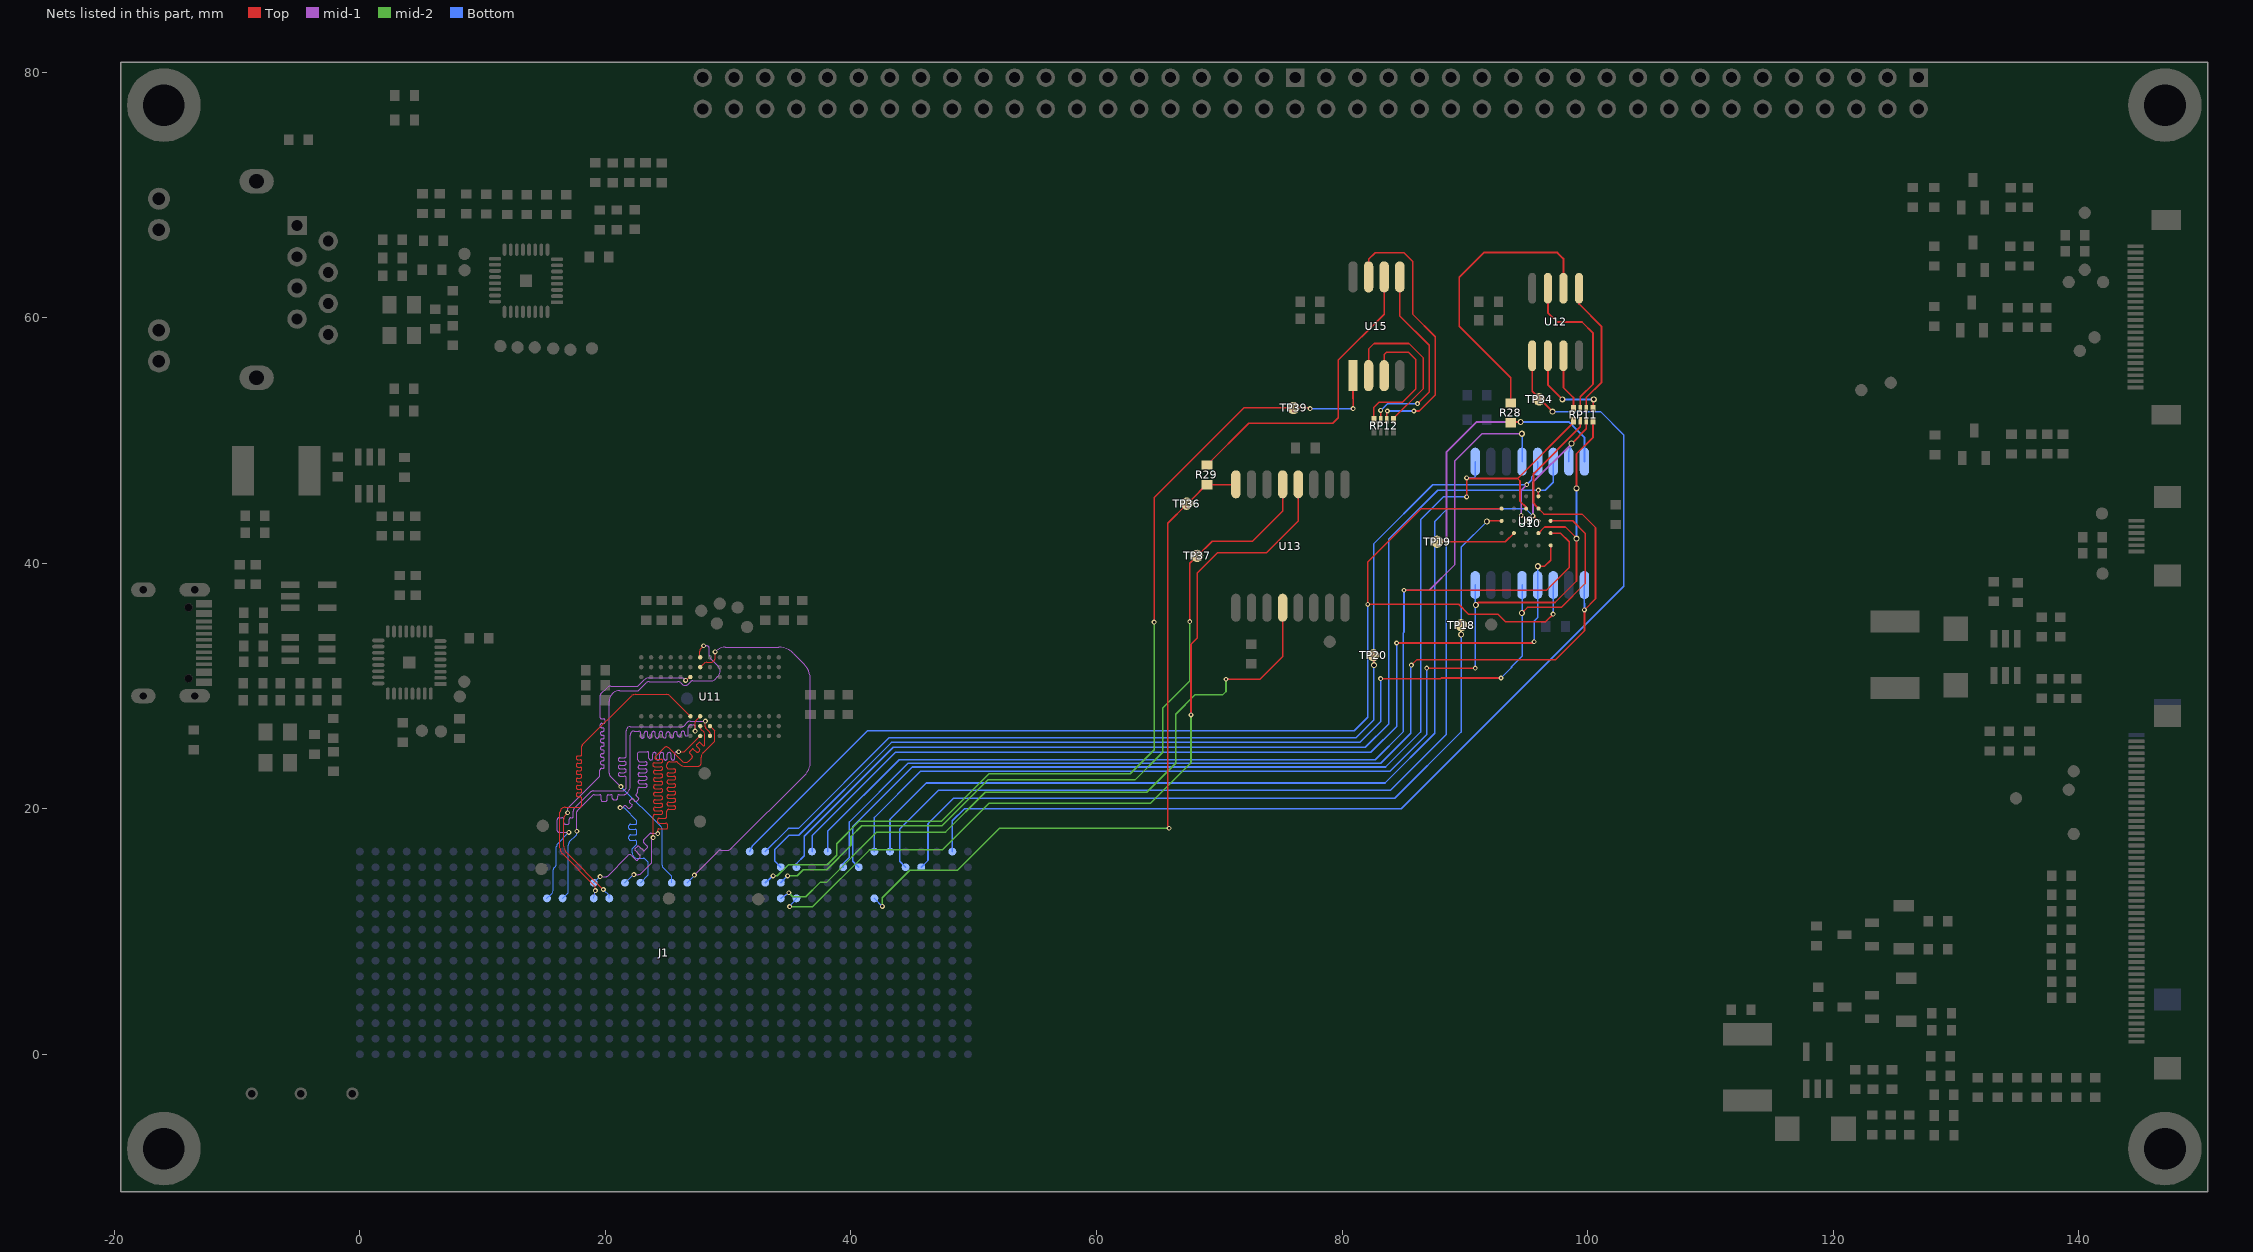
[diagram p0: the nets of this part, all layers, seen from the top]
# Altium PCB MISC105414.PcbDoc (part 8 of 11)
Units mm, origin at the board's own origin, x right, y up, seen from the top; angles counter-clockwise.
Board outline 170 x 92 mm, 6 copper layers (Top, GND, mid-1, mid-2, mid-3, Bottom), stack 1.231 mm thick; 238 components, 304 nets, 1456 pads, 1258 vias.
Unrouted connection lines stored in the file: 57.

## Via types
v1: diameter 0.4, hole 0.2, Top to Bottom, tented top, 618 vias
v2: diameter 0.5, hole 0.3, Top to Bottom, tented top, 522 vias
v3: diameter 0.5, hole 0.3, Top to Bottom, 41 vias
v4: diameter 1, hole 0.5, Top to Bottom, tented top, 36 vias
v5: diameter 0.7, hole 0.4, Top to Bottom, tented top, 34 vias
v6: diameter 1.3, hole 1.3, Top to Bottom, tented top, 3 vias
v7: diameter 4, hole 4, Top to Bottom, tented top, 2 vias
v8: diameter 3.3, hole 3.3, Top to Bottom, tented top, 2 vias

## Nets (pads, with @x,y where several pads share a name; then routed paths per layer and width w, separated by ;. In a path a pad name is that pad's centre, name@x,y a point inside that pad or via, vN(x,y) a via of type N, cw(c..) or ccw(c..) an arc to the next point about the centre after c; other vN are vias at no path point) (continued)
NOR_D6: J1.J12 U13.12 | length 67.1
  Top w0.127: v1(67.7,27.65) 67.7,33.4 68.2,33.9 68.2,39.2 69.85,40.85 73.85,40.85 76.435,43.435 U13.12@76.435,46.425
  mid-2 w0.127: v1(34.998,12.029) 36.886,12.029 41.504,16.648 47.446,16.648 51.246,20.447 64.397,20.447 67.7,23.75 v1(67.7,27.65)
  Bottom w0.127: v1(34.998,12.029) J1.J12@35.56,12.7
NOR_D7: J1.J13 U13.4 | length 56.2
  Top w0.127: v1(70.55,30.55) 73.315,30.55 75.165,32.4 U13.4@75.165,36.375
  mid-2 w0.127: v1(34.943,13.157) 35.265,12.835 36.323,12.835 37.485,13.997 38.006,13.997 42.109,18.1 47.7,18.1 50.947,21.347 64.097,21.347 66.45,23.7 66.45,27.7 68.05,29.3 70.3,29.3 70.55,29.55 v1(70.55,30.55)
  Bottom w0.127: J1.J13@34.29,12.7 v1(34.943,13.157)
NOR_DQS: J1.K13 TP37.1 U13.13 | length 63.8
  Top w0.127: v1(67.6,35.25) 67.6,40 TP37.1@68.2,40.6 68.227,40.6 69.427,41.8 72.715,41.8 75.165,44.25 U13.13@75.165,46.425
  mid-2 w0.127: v1(34.838,14.537) 35.619,14.537 36.124,15.042 38.024,15.042 40.006,17.024 40.006,17.75 40.881,18.625 47.425,18.625 51.147,22.347 63.147,22.347 65.4,24.6 65.4,28.2 67.6,30.4 v1(67.6,35.25)
  Bottom w0.127: J1.K13@34.29,13.97 v1(34.838,14.537)
NOR_SCLK: J1.J7 R29.2 TP36.1 U13.16 | length 59.6
  Top w0.127: v1(65.913,18.415) 65.913,18.489 65.8,18.602 65.8,43.251 67.375,44.825 67.75,45.201 ; TP36.1@67.35,44.85 67.701,45.201 67.75,45.201 ; U13.16@71.355,46.425 71.33,46.4 68.949,46.4 67.75,45.201
  mid-2 w0.127: v1(42.554,12.045) 42.554,12.759 44.79,14.995 48.688,14.995 52.108,18.415 v1(65.913,18.415)
  Bottom w0.127: J1.J7@41.91,12.7 v1(42.554,12.045)
NORE_CS: J1.K14 TP39.1 U15.1 | length 79.2
  Top w0.127: v1(64.7,35.2) 64.7,45.35 72,52.65 TP39.1@76.05,52.65 77.35,52.65 v1(77.4,52.6) ; U15.1@80.895,55.279 80.895,53.407 80.9,53.402 v1(80.9,52.6)
  mid-2 w0.127: v1(33.665,14.534) 33.993,14.534 34.904,15.445 38.068,15.445 38.839,16.216 38.839,17.15 40.664,18.975 47.375,18.975 51.247,22.847 62.747,22.847 64.7,24.8 v1(64.7,35.2)
  Bottom w0.127: J1.K14@33.02,13.97 v1(33.665,14.534) ; v1(77.4,52.6) v1(80.9,52.6)
NORE_D0: RP12.7 U15.5 | length 15.7
  Top w0.127: RP12.7@83.15,51.7 83.15,51.85 v1(83.15,52.45) ; U15.5@84.705,63.321 84.705,60.145 87.1,57.75 87.1,53.95 v1(86.15,53)
  Bottom w0.127: v1(83.15,52.45) 83.7,53 v1(86.15,53)
NORE_D1: RP12.5 U15.2 | length 13.3
  Top w0.127: U15.2@82.165,55.279 82.165,57.45 82.615,57.9 85.45,57.9 86.6,56.75 86.6,54.2 84.2,51.8 RP12.5@84.2,51.7
NORE_D2: RP12.8 U15.3 | length 12
  Top w0.127: RP12.8@82.6,51.7 82.6,52.7 83,53.1 84.9,53.1 86,54.2 86,56.6 85.4,57.2 83.635,57.2 83.435,57 U15.3@83.435,55.279
NORE_D3: RP12.6 U15.7 | length 22.4
  Top w0.127: U15.7@82.165,63.321 82.165,64.755 82.71,65.3 85.05,65.3 85.75,64.6 85.75,60.3 87.6,58.45 87.6,53.702 86.298,52.4 v1(85.85,52.4) ; RP12.6@83.65,51.7 83.65,52.4 v1(83.7,52.4)
  Bottom w0.127: v1(83.7,52.4) v1(85.85,52.4)
NORE_SCLK: R29.1 U15.6 | length 25.3
  Top w0.127: R29.1@69,48 72.4,51.4 79.25,51.4 79.7,51.85 79.7,56.55 83.435,60.285 U15.6@83.435,63.321
PS_CS: J1.L4 TP18.1 U9.A3 | length 70.3
  Top w0.127: v2(89.7,34.2) TP18.1@89.7,34.95 ; v2(91.8,43.4) 91.8,43.45 92.467,43.45 U9.A3@93,43.45
  Bottom w0.127: J1.L4@45.72,15.24 46.275,15.795 46.275,18.775 48.35,20.85 84.3,20.85 89.7,26.25 v2(89.7,34.2) 89.7,41.3 v2(91.8,43.4)
PS_D0: J1.M6 RP11.3 U9.D3 U10.15 | length 87.5
  Top w0.127: v1(95.55,43.85) U9.D3@96,43.45
  Top w0.15: v2(98.7,49.75) 99.9,50.95 RP11.3@99.9,51.6
  mid-1 w0.15: v1(95.55,43.85) 95.55,46.6 v2(98.7,49.75)
  Bottom w0.127: J1.M6@43.18,16.51 43.18,19.14 46.14,22.1 83.5,22.1 87.55,26.15 87.55,43.4 88.6,44.45 94.95,44.45 v1(95.55,43.85)
  Bottom w0.15: U10.15@98.475,48.275 98.475,49.037 v2(98.7,49.75)
PS_D1: J1.M7 RP11.4 U9.D2 U10.8 | length 93.1
  Top w0.127: v1(86.9,31.45) v1(90.85,31.45) ; v2(90.9,36.6) 91.1,36.8 97.35,36.8 99.1,38.55 v2(99.1,42) 99.1,42.05 98.2,42.95 96.5,42.95 U9.D2@96,42.45
  Top w0.15: v2(99.1,46.1) 99.1,48.9 100.45,50.25 RP11.4@100.45,51.6
  Bottom w0.127: J1.M7@41.91,16.51 41.91,19.292 45.668,23.05 83.9,23.05 86.9,26.05 v1(86.9,31.45) ; v1(90.85,31.45) 90.85,34.384 90.855,34.389 v2@90.855,36.6 ; U10.8@90.855,38.225 v2@90.855,36.6 ; v2(90.9,36.6) v2@90.855,36.6
  Bottom w0.15: v2(99.1,42) v2(99.1,46.1)
PS_D2: J1.L8 RP11.1 U9.C4 U10.9 | length 91.8
  Top w0.127: v1(90.15,45.4) v1(90.15,46.95) 90.2,46.9 94.3,46.9 94.5,46.7 94.5,45.05 95,44.55 U9.C4@95,44.45
  Top w0.15: 94.3,46.9 98.85,51.45 RP11.1@98.85,51.6
  Bottom w0.127: J1.L8@40.64,15.24 40.156,15.723 40.156,18.556 45,23.4 83.55,23.4 86.4,26.25 86.4,43.55 88.25,45.4 v1(90.15,45.4) ; v1(90.15,46.95) 90.75,46.95 90.855,47.05 U10.9@90.855,48.275
PS_D3: J1.L9 RP11.2 U9.D4 U10.1 | length 98.4
  Top w0.127: v1(85.65,31.7) 86.1,32.15 97.4,32.15 99.75,34.5 v1(99.75,36.2) 100.65,37.1 100.65,42.9 99.55,44 96.45,44 U9.D4@96,44.45
  Top w0.15: U9.D4@96,44.45 95.6,44.9 95.6,47.3 99.4,51.1 RP11.2@99.4,51.6
  Bottom w0.127: J1.L9@39.37,15.24 39.37,15.533 39.878,16.041 39.878,18.928 44.65,23.7 83.15,23.7 85.6,26.15 85.6,31.65 v1(85.65,31.7) ; U10.1@99.745,38.225 99.745,36.744 99.75,36.738 v1(99.75,36.2)
PS_D4: J1.L12 U9.D5 U10.14 | length 86.7
  Top w0.127: U9.D5@96,45.45 v1(96,45.95)
  Bottom w0.127: J1.L12@35.56,15.24 35.56,15.533 36.2,16.173 36.2,17.754 43.446,25 81.9,25 83.8,26.9 83.8,41.95 87.8,45.95 v1(96,45.95) 96.55,45.95 97.205,46.605 U10.14@97.205,48.275
PS_D5: J1.L13 U9.E3 U10.5 | length 90.4
  Top w0.127: v1(83.15,30.6) 88.025,30.6 88.075,30.65 v1(92.95,30.65) ; v2(94.65,35.95) 95.1,36.4 97.85,36.4 99.8,38.35 99.8,42.45 98.8,43.45 U9.E3@97,43.45
  Bottom w0.127: J1.L13@34.29,15.24 33.806,15.723 33.806,16.71 34.946,17.85 35.75,17.85 43.3,25.4 81.45,25.4 83.15,27.1 v1(83.15,30.6) ; v1(92.95,30.65) 93.807,31.507 93.807,31.557 94.665,32.415 v2@94.665,35.95 ; v2(94.65,35.95) v2@94.665,35.95 ; U10.5@94.665,38.225 v2@94.665,35.95
PS_D6: J1.M10 U9.E2 U10.12 | length 103.7
  Top w0.127: v1(85.05,37.8) 96.65,37.8 98.5,39.65 98.5,41.75 97.8,42.45 U9.E2@97,42.45
  mid-1 w0.127: v1(85.05,37.8) 87.1,37.8 89.2,39.9 89.2,48.35 91.4,50.55 v2(94.65,50.55)
  Bottom w0.127: J1.M10@38.1,16.51 38.1,18.175 43.925,24 82.7,24 85,26.3 85,34.35 85.05,34.4 v1(85.05,37.8) ; v2(94.65,50.55) 94.665,50.535 U10.12@94.665,48.275
PS_D7: J1.M11 U9.E1 U10.4 | length 79.4
  Top w0.127: v1(84.45,33.5) 95.55,33.5 v1(95.65,33.6) ; v2(95.95,39.75) 96.5,39.75 97,40.25 U9.E1@97,41.45
  Bottom w0.127: J1.M11@36.83,16.51 36.83,17.8 43.63,24.6 82.35,24.6 84.45,26.7 v1(84.45,33.5) ; v1(95.65,33.6) 95.65,35.299 95.935,35.583 95.935,38.987 v2(95.95,39.75)
PS_DQS: J1.M14 TP20.1 U9.C3 U10.13 | length 89.1
  Top w0.127: TP20.1@82.55,32.5 v2(82.6,31.7) ; v1(94.6,43.9) U9.C3@95,43.45
  mid-1 w0.127: v1(94.6,43.9) 94.6,45.95 v1(95.05,46.4)
  Bottom w0.127: J1.M14@33.02,16.51 34.91,18.4 35.725,18.4 43.125,25.8 81.15,25.8 82.6,27.25 v2(82.6,31.7) 82.6,41.6 87.4,46.4 v1(95.05,46.4) 95.45,46.8 95.45,47.028 95.935,47.513 U10.13@95.935,48.275
PS_RSTN: J1.M15 U9.A4 U10.3 | length 98.6
  Top w0.127: U9.A4@93,44.45 86.45,44.45 82.1,40.1 v1(82.1,36.65) 89.5,36.65 90.3,35.85 92.7,35.85 93.3,35.25 96.6,35.25 v1(97.2,35.85)
  Bottom w0.127: J1.M15@31.75,16.51 31.969,16.975 41.343,26.35 81,26.35 82.1,27.45 v1(82.1,36.65) ; v1(97.2,35.85) 97.2,36.564 97.205,36.568 U10.3@97.205,38.225
PS_SCLK: J1.L5 R28.2 TP19.1 U9.B2 U10.16 | length 96.2
  Top w0.127: v1(88.5,41.75) 93.3,41.75 U9.B2@94,42.45
  Top w0.15: TP19.1@87.75,41.75 v1(88.5,41.75) ; R28.2@93.75,51.45 93.75,51.5 v2(94.55,51.5)
  mid-1 w0.15: v1(88.5,41.75) 88.5,49.05 90.95,51.5 v2(94.55,51.5)
  Bottom w0.127: J1.L5@44.45,15.24 43.966,15.723 43.966,18.341 47.125,21.5 83.95,21.5 88.5,26.05 v1(88.5,41.75)
  Bottom w0.15: v2(94.55,51.5) 98.5,51.5 99.745,50.255 U10.16@99.745,48.275
PSE_CS: J1.M2 TP34.1 U12.1 | length 89.4
  Top w0.15: U12.1@95.495,56.9 95.495,54.005 TP34.1@96.15,53.35 ; TP34.1@96.05,53.35 TP34.1@96.15,53.35 ; v2(97.15,52.35) 96.5,53 TP34.1@96.15,53.35
  Bottom w0.127: J1.M2@48.26,16.51 48.26,19.019 49.241,20 84.825,20 102.95,38.125 102.95,50.45 101.05,52.35 v2(97.15,52.35)
PSE_D0: RP11.6 U12.5 | length 11.1
  Top w0.15: U12.5@99.305,62.4 99.305,61.122 101.15,59.277 101.15,54.75 99.9,53.5 RP11.6@99.9,52.6
PSE_D1: RP11.5 U12.2 | length 7.4
  Top w0.15: U12.2@96.765,56.9 96.765,54.535 v2(97.95,53.35) ; RP11.5@100.45,52.6 100.463,52.6 100.463,53.35 v2(100.5,53.35)
  Bottom w0.15: v2(97.95,53.35) v2(100.5,53.35)
PSE_D2: RP11.8 U12.3 | length 4.6
  Top w0.15: U12.3@98.035,56.9 98.035,54.315 98.85,53.5 RP11.8@98.85,52.6
PSE_D3: RP11.7 U12.7 | length 13
  Top w0.15: U12.7@96.765,62.4 96.765,60.4 97.515,59.65 99.55,59.65 100.45,58.75 100.45,54.6 99.4,53.55 RP11.7@99.4,52.6
PSE_SCLK: R28.1 U12.6 | length 23.9
  Top w0.15: R28.1@93.75,53.05 93.75,55.1 89.55,59.3 89.55,63.3 91.55,65.3 97.55,65.3 98.035,64.815 U12.6@98.035,62.4
SDR_A0: J1.K19 U11.G8 | length 32.5
  Top w0.1: U11.G8@27.72,31.533 28.017,31.83 cw(c28.253,31.595) 28.253,31.928 28.511,31.928 ccw(c28.511,32.41) 28.852,32.069 28.853,32.07 ccw(c28.657,32.267) 28.935,32.267 v1(28.935,32.781)
  mid-1 w0.1: v1(27.25,14.6) 29.204,16.554 cw(c29.397,16.362) 29.397,16.634 30.017,16.634 ccw(c30.017,16.854) 30.172,16.699 36.34,22.866 ccw(c35.522,23.684) 36.679,23.684 36.679,30.606 ccw(c35.03,30.606) 36.196,31.772 35.286,32.681 ccw(c34.103,31.498) 34.103,33.171 29.773,33.171 ccw(c29.773,32.091) 29.009,32.855 v1(28.935,32.781)
  Bottom w0.1: J1.K19@26.67,13.97 27.25,14.55 v1(27.25,14.6) v1@27.3,14.6
SDR_A1: J1.K20 U11.G9 | length 31.2
  Top w0.1: U11.G9@27.72,32.333 27.679,32.333 27.679,32.845 cw(c27.962,32.845) 27.762,33.044 v1(27.993,33.275)
  mid-1 w0.1: v1(21.266,21.808) 20.369,22.705 cw(c20.536,22.872) 20.3,22.872 20.3,28.759 cw(c21.154,28.759) 21.154,29.613 22.69,29.613 23.338,30.261 cw(c23.554,30.046) 23.554,30.351 25.91,30.351 cw(c25.91,30.032) 26.135,30.257 26.247,30.146 ccw(c26.449,30.348) 26.449,30.062 26.573,30.062 ccw(c26.573,30.254) 26.709,30.118 26.94,30.349 cw(c27.114,30.176) 27.114,30.421 28.619,30.421 ccw(c28.619,30.888) 28.949,30.558 29.166,30.776 ccw(c28.73,31.212) 29.347,31.212 ccw(c28.73,31.212) 29.166,31.648 28.594,32.22 cw(c28.893,32.518) 28.471,32.518 28.471,33.023 ccw(c28.219,33.023) 28.219,33.275 v1(27.993,33.275)
  Bottom w0.1: v1(21.266,21.808) 24.513,18.561 cw(c24.266,18.315) 24.615,18.315 24.615,15.418 ccw(c24.918,15.418) 24.703,15.204 25.365,14.543 cw(c25.28,14.458) 25.4,14.458 J1.K20@25.4,13.97
SDR_A2: J1.J24 U11.F7 | length 30.5
  Top w0.1: v1(16.923,19.672) 16.723,19.472 ccw(c17.03,19.164) 16.596,19.164 16.596,16.948 ccw(c17.275,16.948) 16.795,16.467 v1(19.84,13.422) ; v1(26.534,30.451) U11.F7@26.92,30.733
  mid-1 w0.1: v1(16.923,19.672) 16.923,20.007 cw(c16.987,20.007) 16.941,20.052 19.555,22.666 19.555,23.141 cw(c19.705,23.141) 19.705,23.291 19.774,23.291 ccw(c19.774,23.441) 19.924,23.441 ccw(c19.774,23.441) 19.774,23.591 19.733,23.591 cw(c19.733,23.741) 19.583,23.741 cw(c19.733,23.741) 19.733,23.891 19.774,23.891 ccw(c19.774,24.041) 19.924,24.041 ccw(c19.774,24.041) 19.774,24.191 19.733,24.191 cw(c19.733,24.341) 19.583,24.341 cw(c19.733,24.341) 19.733,24.491 19.774,24.491 ccw(c19.774,24.641) 19.924,24.641 ccw(c19.774,24.641) 19.774,24.791 19.733,24.791 cw(c19.733,24.941) 19.583,24.941 cw(c19.733,24.941) 19.733,25.091 19.774,25.091 ccw(c19.774,25.241) 19.924,25.241 ccw(c19.774,25.241) 19.774,25.391 19.733,25.391 cw(c19.733,25.541) 19.583,25.541 cw(c19.733,25.541) 19.733,25.691 19.774,25.691 ccw(c19.774,25.841) 19.924,25.841 ccw(c19.774,25.841) 19.774,25.991 19.733,25.991 cw(c19.733,26.141) 19.583,26.141 cw(c19.733,26.141) 19.733,26.291 19.774,26.291 ccw(c19.774,26.441) 19.924,26.441 ccw(c19.774,26.441) 19.774,26.591 19.733,26.591 cw(c19.733,26.741) 19.583,26.741 19.583,26.85 cw(c19.688,26.85) 19.688,26.955 19.849,26.955 ccw(c19.849,27.073) 19.966,27.073 19.966,27.221 ccw(c19.864,27.221) 19.864,27.324 19.672,27.324 cw(c19.672,27.413) 19.583,27.413 19.583,29.241 cw(c19.74,29.241) 19.629,29.352 20.133,29.856 cw(c20.44,29.55) 20.44,29.983 22.578,29.983 ccw(c22.578,30.118) 22.673,30.023 23.173,30.522 cw(c23.485,30.21) 23.485,30.652 26.234,30.652 cw(c26.234,30.431) 26.39,30.587 26.539,30.438 v1(26.534,30.451)
  Bottom w0.1: v1(19.84,13.422) 20.32,12.942 J1.J24@20.32,12.7
SDR_A3: J1.J25 U11.F3 | length 30.6
  Top w0.1: v1(19.19,13.334) 19.19,13.646 16.479,16.358 cw(c16.921,16.8) 16.295,16.8 16.295,19.697 cw(c16.72,19.697) 16.72,20.122 17.873,20.122 ccw(c17.873,20.316) 18.068,20.316 18.068,20.848 ccw(c17.918,20.848) 17.918,20.998 17.759,20.998 cw(c17.759,21.148) 17.609,21.148 cw(c17.759,21.148) 17.759,21.298 17.938,21.298 ccw(c17.938,21.448) 18.088,21.448 ccw(c17.938,21.448) 17.938,21.598 17.759,21.598 cw(c17.759,21.748) 17.609,21.748 cw(c17.759,21.748) 17.759,21.898 17.938,21.898 ccw(c17.938,22.048) 18.088,22.048 ccw(c17.938,22.048) 17.938,22.198 17.759,22.198 cw(c17.759,22.348) 17.609,22.348 cw(c17.759,22.348) 17.759,22.498 17.938,22.498 ccw(c17.938,22.648) 18.088,22.648 ccw(c17.938,22.648) 17.938,22.798 17.759,22.798 cw(c17.759,22.948) 17.609,22.948 cw(c17.759,22.948) 17.759,23.098 17.938,23.098 ccw(c17.938,23.248) 18.088,23.248 ccw(c17.938,23.248) 17.938,23.398 17.759,23.398 cw(c17.759,23.548) 17.609,23.548 cw(c17.759,23.548) 17.759,23.698 17.938,23.698 ccw(c17.938,23.848) 18.088,23.848 ccw(c17.938,23.848) 17.938,23.998 17.759,23.998 cw(c17.759,24.148) 17.609,24.148 cw(c17.759,24.148) 17.759,24.298 17.941,24.298 ccw(c17.941,24.448) 18.091,24.448 18.091,25.111 cw(c18.212,25.111) 18.126,25.197 22.113,29.184 cw(c22.416,28.88) 22.416,29.31 24.996,29.31 cw(c24.996,28.952) 25.248,29.205 U11.F3@26.92,27.533
  Bottom w0.1: J1.J25@19.05,12.7 v1(19.19,13.334)
SDR_A4: J1.K22 U11.G1 | length 31.6
  Top w0.1: v1(25.966,24.642) 26.429,24.642 U11.G1@27.72,25.933
  mid-1 w0.1: v1(21.201,20.086) 21.342,20.086 ccw(c21.342,20.179) 21.408,20.113 21.528,20.233 cw(c21.601,20.16) 21.674,20.233 21.853,20.055 ccw(c21.922,20.124) 21.991,20.055 22.169,20.233 ; 22.085,20.774 21.97,20.659 ccw(c22.045,20.584) 21.939,20.584 ccw(c22.045,20.584) 21.97,20.509 22.169,20.31 ; 22.085,20.774 cw(c22.167,20.691) 22.249,20.774 22.396,20.627 ccw(c22.48,20.71) 22.563,20.627 22.706,20.77 ccw(c22.653,20.822) 22.727,20.822 ccw(c22.653,20.822) 22.706,20.874 22.515,21.065 cw(c22.584,21.134) 22.486,21.134 cw(c22.584,21.134) 22.515,21.204 22.577,21.265 ccw(c22.482,21.36) 22.616,21.36 22.616,21.592 cw(c22.766,21.592) 22.766,21.742 23.253,21.742 ccw(c23.253,21.892) 23.403,21.892 ccw(c23.253,21.892) 23.253,22.042 22.803,22.042 cw(c22.803,22.192) 22.653,22.192 cw(c22.803,22.192) 22.803,22.342 23.253,22.342 ccw(c23.253,22.492) 23.403,22.492 ccw(c23.253,22.492) 23.253,22.642 22.803,22.642 cw(c22.803,22.792) 22.653,22.792 cw(c22.803,22.792) 22.803,22.942 23.253,22.942 ccw(c23.253,23.092) 23.403,23.092 ccw(c23.253,23.092) 23.253,23.242 22.803,23.242 cw(c22.803,23.392) 22.653,23.392 cw(c22.803,23.392) 22.803,23.542 23.253,23.542 ccw(c23.253,23.692) 23.403,23.692 ccw(c23.253,23.692) 23.253,23.842 22.803,23.842 cw(c22.803,23.992) 22.653,23.992 22.653,24.552 22.755,24.653 23.393,24.653 cw(c23.393,24.503) 23.543,24.503 23.543,24.121 ccw(c23.693,24.121) 23.843,24.121 23.843,24.436 cw(c23.993,24.436) 24.143,24.436 24.143,24.121 ccw(c24.293,24.121) 24.443,24.121 24.443,24.436 cw(c24.593,24.436) 24.743,24.436 24.743,24.121 ccw(c24.893,24.121) 25.043,24.121 25.043,24.436 cw(c25.193,24.436) 25.343,24.436 25.343,24.121 ccw(c25.493,24.121) 25.643,24.121 25.643,24.513 cw(c25.772,24.513) 25.772,24.642 v1(25.966,24.642) ; 22.169,20.233 ccw(c22.13,20.272) 22.185,20.272 ccw(c22.13,20.272) 22.169,20.31
  Bottom w0.1: v1(21.201,20.086) 21.416,20.086 cw(c21.416,19.879) 21.562,20.025 22.504,19.083 cw(c22.37,18.949) 22.56,18.949 22.56,18.849 cw(c22.447,18.849) 22.447,18.736 22.047,18.736 ccw(c22.047,18.604) 21.915,18.604 21.915,18.415 ccw(c22.017,18.415) 22.017,18.312 22.434,18.312 cw(c22.434,18.186) 22.56,18.186 22.56,17.983 cw(c22.447,17.983) 22.447,17.87 22.061,17.87 ccw(c22.061,17.724) 21.915,17.724 21.915,17.571 ccw(c22.065,17.571) 22.065,17.422 22.427,17.422 cw(c22.427,17.288) 22.56,17.288 22.56,17.226 cw(c22.305,17.226) 22.485,17.046 22.18,16.741 22.18,16.408 ccw(c22.613,16.408) 22.613,15.975 23.085,15.975 cw(c23.085,15.814) 23.2,15.928 23.423,15.704 cw(c23.238,15.519) 23.5,15.519 23.5,14.61 J1.K22@22.86,13.97
SDR_A5: J1.K23 U11.G2 | length 30.4
  Top w0.1: v1(23.889,17.647) 23.889,19.389 cw(c24.039,19.389) 24.039,19.539 24.52,19.539 ccw(c24.52,19.689) 24.67,19.689 ccw(c24.52,19.689) 24.52,19.839 24.061,19.839 cw(c24.061,19.989) 23.911,19.989 cw(c24.061,19.989) 24.061,20.139 24.52,20.139 ccw(c24.52,20.289) 24.67,20.289 ccw(c24.52,20.289) 24.52,20.439 24.061,20.439 cw(c24.061,20.589) 23.911,20.589 cw(c24.061,20.589) 24.061,20.739 24.52,20.739 ccw(c24.52,20.889) 24.67,20.889 ccw(c24.52,20.889) 24.52,21.039 24.061,21.039 cw(c24.061,21.189) 23.911,21.189 cw(c24.061,21.189) 24.061,21.339 24.52,21.339 ccw(c24.52,21.489) 24.67,21.489 ccw(c24.52,21.489) 24.52,21.639 24.061,21.639 cw(c24.061,21.789) 23.911,21.789 cw(c24.061,21.789) 24.061,21.939 24.52,21.939 ccw(c24.52,22.089) 24.67,22.089 ccw(c24.52,22.089) 24.52,22.239 24.061,22.239 cw(c24.061,22.389) 23.911,22.389 cw(c24.061,22.389) 24.061,22.539 24.52,22.539 ccw(c24.52,22.689) 24.67,22.689 ccw(c24.52,22.689) 24.52,22.839 24.061,22.839 cw(c24.061,22.989) 23.911,22.989 cw(c24.061,22.989) 24.061,23.139 24.52,23.139 ccw(c24.52,23.289) 24.67,23.289 ccw(c24.52,23.289) 24.52,23.439 23.994,23.439 cw(c23.994,23.589) 23.844,23.589 cw(c23.994,23.589) 23.994,23.739 24.52,23.739 ccw(c24.52,23.889) 24.67,23.889 ccw(c24.52,23.889) 24.52,24.039 24.153,24.039 cw(c24.153,24.161) 24.031,24.161 cw(c24.153,24.161) 24.067,24.247 24.777,24.958 cw(c24.966,24.769) 25.155,24.958 26.201,23.911 ccw(c26.519,24.23) 26.838,23.911 27.05,24.123 ccw(c26.941,24.232) 27.095,24.232 ccw(c26.941,24.232) 27.05,24.341 26.858,24.533 cw(c26.911,24.586) 26.836,24.586 cw(c26.911,24.586) 26.858,24.64 27.082,24.864 cw(c27.12,24.825) 27.159,24.864 ; 27.159,24.864 27.382,24.641 ccw(c27.489,24.748) 27.596,24.641 27.667,24.712 ccw(c27.595,24.785) 27.698,24.785 ccw(c27.595,24.785) 27.667,24.858 27.433,25.092 cw(c27.498,25.157) 27.406,25.157 cw(c27.498,25.157) 27.433,25.222 27.592,25.381 cw(c27.65,25.324) 27.707,25.381 27.923,25.165 ccw(c28.001,25.242) 28.11,25.242 28.11,26.001 ccw(c27.723,26.001) 27.997,26.275 27.78,26.492 cw(c27.925,26.637) 27.72,26.637 U11.G2@27.72,26.733
  mid-1 w0.1: v1(22.317,14.641) 22.676,14.641 ccw(c22.676,14.994) 22.925,14.744 23.734,15.554 ccw(c23.625,15.663) 23.78,15.663 23.78,17.538 v1(23.889,17.647)
  Bottom w0.1: J1.K23@21.59,13.97 22.137,14.517 v1(22.317,14.641)
SDR_A6: J1.J27 U11.G3 | length 31.5
  Top w0.1: v1(27.302,26.332) 27.302,27.052 cw(c27.452,27.052) 27.346,27.158 U11.G3@27.72,27.533
  mid-1 w0.1: v1(17.672,18.167) 17.672,19.753 cw(c17.807,19.753) 17.712,19.849 18.959,21.096 cw(c19.107,20.948) 19.107,21.157 19.549,21.157 cw(c19.549,21.063) 19.643,21.063 19.643,20.729 ccw(c19.771,20.729) 19.771,20.601 19.995,20.601 ccw(c19.995,20.748) 20.141,20.748 20.141,21.059 cw(c20.239,21.059) 20.239,21.157 20.446,21.157 cw(c20.446,21.042) 20.562,21.042 20.562,20.859 ccw(c20.67,20.859) 20.67,20.751 20.895,20.751 ccw(c20.895,20.851) 20.994,20.851 20.994,21.037 cw(c21.114,21.037) 21.114,21.157 21.521,21.157 ccw(c21.521,21.392) 21.687,21.226 21.862,21.401 ccw(c21.505,21.758) 22.01,21.758 22.01,25.997 cw(c22.345,25.997) 22.345,26.332 22.715,26.332 cw(c22.715,26.182) 22.865,26.182 22.865,25.907 ccw(c23.015,25.907) 23.165,25.907 23.165,26.144 cw(c23.315,26.144) 23.465,26.144 23.465,25.907 ccw(c23.615,25.907) 23.765,25.907 23.765,26.144 cw(c23.915,26.144) 24.065,26.144 24.065,25.907 ccw(c24.215,25.907) 24.365,25.907 24.365,26.144 cw(c24.515,26.144) 24.665,26.144 24.665,25.923 ccw(c24.815,25.923) 24.965,25.923 24.965,26.108 cw(c25.115,26.108) 25.265,26.108 25.265,25.923 ccw(c25.415,25.923) 25.565,25.923 25.565,26.135 cw(c25.715,26.135) 25.865,26.135 25.865,26.016 ccw(c26.015,26.016) 26.165,26.016 26.165,26.164 cw(c26.315,26.164) 26.465,26.164 26.465,26.077 ccw(c26.615,26.077) 26.765,26.077 26.765,26.627 cw(c26.903,26.627) 26.805,26.725 26.879,26.798 cw(c26.973,26.704) 26.973,26.837 27.203,26.837 cw(c27.203,26.739) 27.302,26.739 v1(27.302,26.332)
  Bottom w0.1: J1.J27@16.51,12.7 16.984,13.174 16.984,17.033 cw(c17.413,17.033) 17.11,17.336 17.608,17.834 ccw(c17.451,17.99) 17.672,17.99 v1(17.672,18.167)
SDR_A7: J1.J28 U11.H1 | length 31.8
  Top w0.1: v1(28.137,27.138) 28.137,26.677 ccw(c28.337,26.677) 28.195,26.535 28.479,26.251 cw(c28.381,26.152) 28.52,26.152 U11.H1@28.52,25.933
  mid-1 w0.1: v1(17.031,18.072) 16.226,18.072 cw(c16.226,18.216) 16.081,18.216 16.081,19.123 cw(c16.236,19.123) 16.236,19.278 16.456,19.278 cw(c16.456,19.13) 16.604,19.13 16.604,18.867 ccw(c16.721,18.867) 16.721,18.751 16.959,18.751 ccw(c16.959,18.841) 17.05,18.841 17.05,19.137 cw(c17.169,19.137) 17.169,19.255 17.279,19.255 ccw(c17.279,19.349) 17.372,19.349 17.372,19.816 cw(c17.664,19.816) 17.458,20.022 18.803,21.367 cw(c19.019,21.151) 19.019,21.457 21.39,21.457 ccw(c21.39,21.702) 21.563,21.529 21.654,21.619 ccw(c21.539,21.733) 21.701,21.733 21.701,22.502 ccw(c21.551,22.502) 21.551,22.652 21.198,22.652 cw(c21.198,22.802) 21.048,22.802 cw(c21.198,22.802) 21.198,22.952 21.547,22.952 ccw(c21.547,23.102) 21.697,23.102 ccw(c21.547,23.102) 21.547,23.252 21.198,23.252 cw(c21.198,23.402) 21.048,23.402 cw(c21.198,23.402) 21.198,23.552 21.547,23.552 ccw(c21.547,23.702) 21.697,23.702 ccw(c21.547,23.702) 21.547,23.852 21.198,23.852 cw(c21.198,24.002) 21.048,24.002 cw(c21.198,24.002) 21.198,24.152 21.547,24.152 ccw(c21.547,24.302) 21.697,24.302 21.697,26.352 cw(c22.033,26.352) 22.033,26.688 26.234,26.688 ccw(c26.234,26.954) 26.422,26.766 26.724,27.068 cw(c26.892,26.9) 26.892,27.138 v1(28.137,27.138)
  Bottom w0.1: J1.J28@15.24,12.7 15.622,13.082 ccw(c15.319,13.386) 15.748,13.386 15.748,15.046 cw(c15.983,15.046) 15.817,15.212 15.942,15.337 ccw(c15.768,15.511) 16.014,15.511 16.014,16.913 cw(c16.356,16.913) 16.114,17.155 v1(17.031,18.072)
SDR_A8: J1.K25 U11.H2 | length 30.9
  Top w0.1: v1(24.263,17.981) 24.263,18.262 cw(c24.364,18.262) 24.364,18.363 24.962,18.363 ccw(c24.962,18.464) 25.063,18.464 25.063,18.691 ccw(c24.924,18.691) 24.924,18.829 24.393,18.829 cw(c24.393,18.96) 24.263,18.96 24.263,19.113 cw(c24.388,19.113) 24.388,19.238 24.873,19.238 ccw(c24.873,19.37) 25.006,19.37 25.006,19.794 cw(c25.156,19.794) 25.156,19.944 25.58,19.944 ccw(c25.58,20.094) 25.73,20.094 ccw(c25.58,20.094) 25.58,20.244 25.16,20.244 cw(c25.16,20.394) 25.01,20.394 cw(c25.16,20.394) 25.16,20.544 25.58,20.544 ccw(c25.58,20.694) 25.73,20.694 ccw(c25.58,20.694) 25.58,20.844 25.16,20.844 cw(c25.16,20.994) 25.01,20.994 cw(c25.16,20.994) 25.16,21.144 25.58,21.144 ccw(c25.58,21.294) 25.73,21.294 ccw(c25.58,21.294) 25.58,21.444 25.16,21.444 cw(c25.16,21.594) 25.01,21.594 cw(c25.16,21.594) 25.16,21.744 25.58,21.744 ccw(c25.58,21.894) 25.73,21.894 ccw(c25.58,21.894) 25.58,22.044 25.16,22.044 cw(c25.16,22.194) 25.01,22.194 cw(c25.16,22.194) 25.16,22.344 25.58,22.344 ccw(c25.58,22.494) 25.73,22.494 ccw(c25.58,22.494) 25.58,22.644 25.16,22.644 cw(c25.16,22.794) 25.01,22.794 cw(c25.16,22.794) 25.16,22.944 25.58,22.944 ccw(c25.58,23.094) 25.73,23.094 ccw(c25.58,23.094) 25.58,23.244 25.16,23.244 cw(c25.16,23.394) 25.01,23.394 25.01,23.599 cw(c25.243,23.599) 25.243,23.832 25.736,23.832 cw(c25.736,23.602) 25.899,23.764 26.044,23.62 ccw(c26.384,23.96) 26.384,23.479 27.573,23.479 ccw(c27.573,23.699) 27.793,23.699 27.793,24.188 cw(c28.338,24.188) 27.952,24.573 28.889,25.51 28.889,26.364 U11.H2@28.52,26.733
  mid-1 w0.1: v1(19.568,14.476) 20.086,14.476 ccw(c20.086,14.602) 20.175,14.513 21.879,16.217 cw(c21.987,16.109) 22.095,16.217 22.463,15.848 ccw(c22.557,15.942) 22.651,15.848 22.809,16.006 ccw(c22.698,16.117) 22.855,16.117 ccw(c22.698,16.117) 22.809,16.229 22.428,16.61 cw(c22.506,16.688) 22.396,16.688 cw(c22.506,16.688) 22.428,16.766 22.573,16.911 cw(c22.671,16.813) 22.768,16.911 23.07,16.609 ; 23.07,16.609 ccw(c23.131,16.67) 23.192,16.609 ; 23.192,16.609 23.425,16.842 ccw(c23.372,16.895) 23.447,16.895 ccw(c23.372,16.895) 23.425,16.948 23.125,17.248 cw(c23.231,17.355) 23.08,17.355 cw(c23.231,17.355) 23.124,17.462 23.618,17.956 cw(c23.746,17.828) 23.746,18.009 24.235,18.009 v1(24.263,17.981)
  Bottom w0.1: J1.K25@19.05,13.97 19.562,14.482 v1(19.568,14.476)